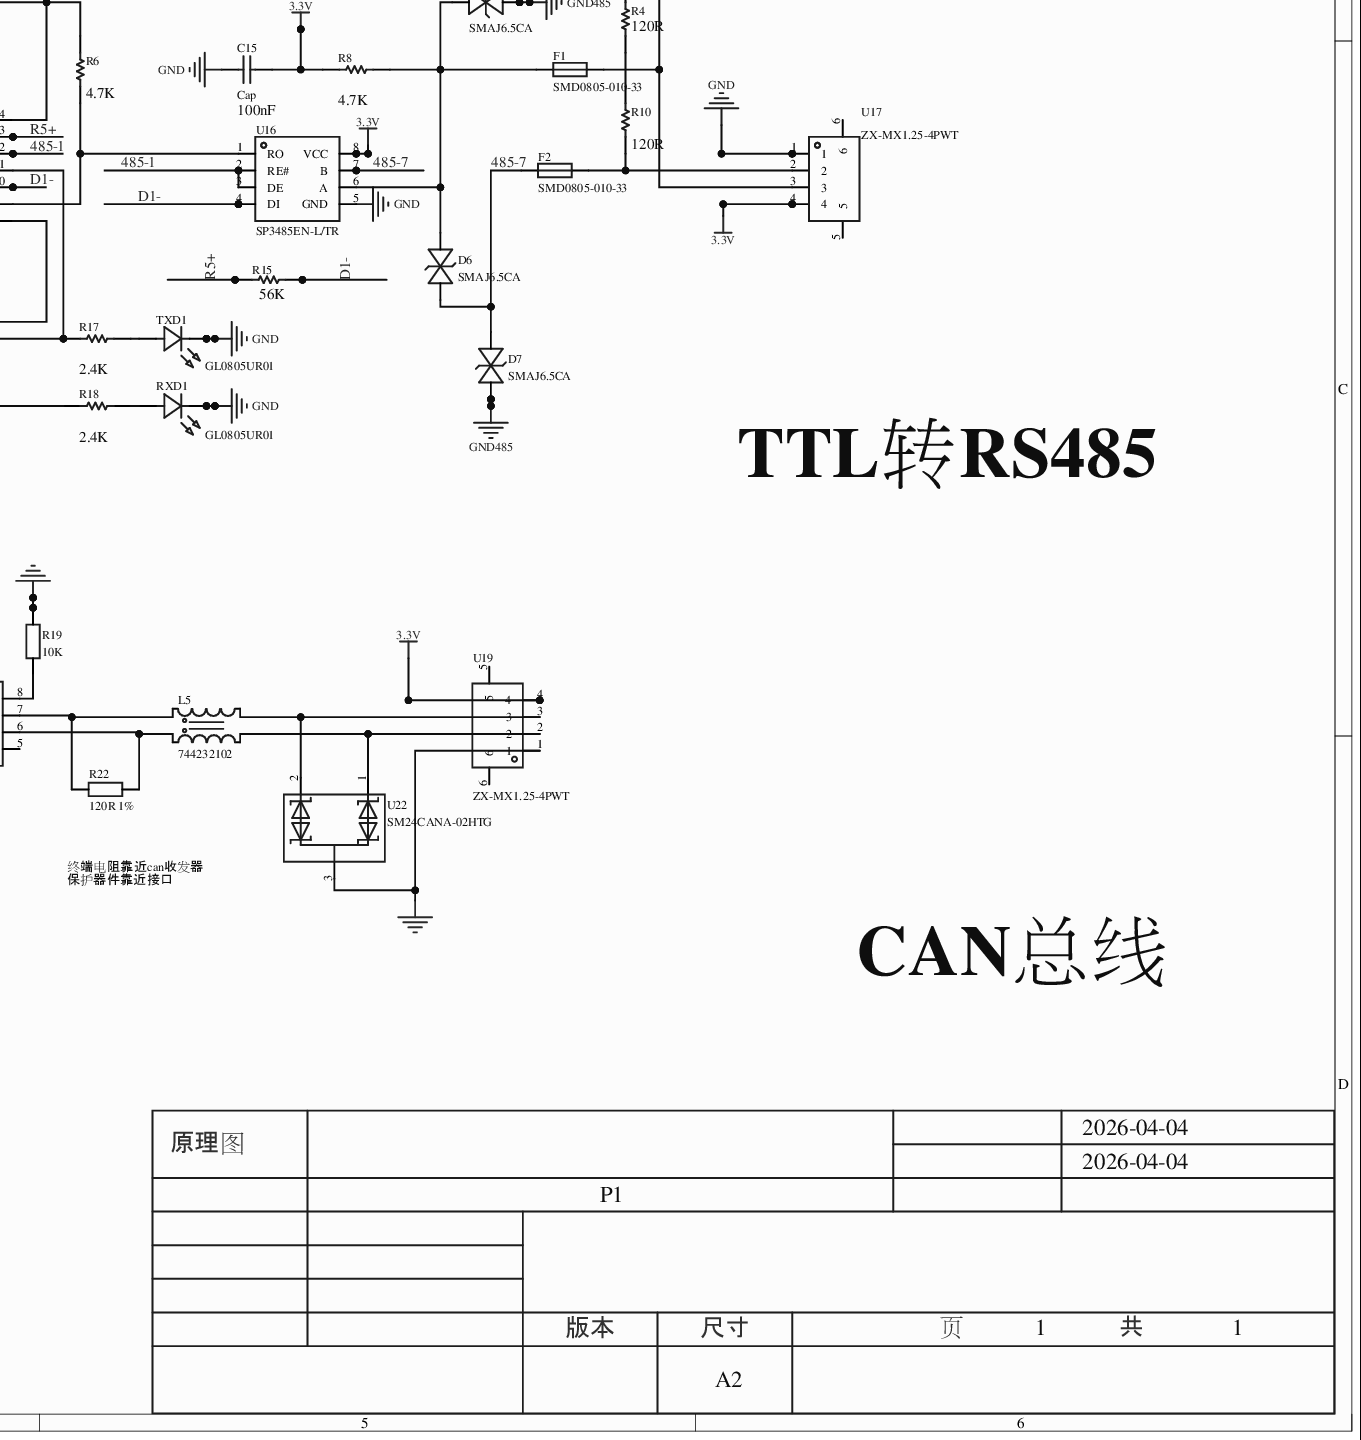
[diagram p0: MISC51972-3.schdoc, bottom right]
# Altium project MISC51972-2.PrjPcb (part 3 of 3)

## Sheet MISC51972-3.schdoc (continued)

### Library data of the parts
C1 C3 C4 C6-C8 = CAP_0402: SymbolName: CapAcitance; ConvertToPcb: yes; ModelId: 36a51122f27c49738f86b3bfa98863e0; ModelName: C0402_L1.0-W0.5-H0.5; ModelTransform: 39.37,19.685,0,0,0,0,0,0,0; Device: CAP_0402; FootprintName: C0402; AddInBom: yes; Supplier Footprint: 0402; Value: 100nF
C2 C5 C9-C14 C16-C20 C27 C28 C35 C36 = CAP_0603: SymbolName: CapAcitance; ConvertToPcb: yes; ModelId: ac125912035d415993ca9572d50418b1; ModelName: C0603_L1.6-W0.8-H0.8; ModelTransform: 62.992,31.496,0,0,0,0,0,0,0; Device: CAP_0603; FootprintName: C0402; AddInBom: yes; Supplier Footprint: 0603
  C2 C5 C11-C14 C16-C20: Value: 100nF
  C9 C10: Value: 12pF
  C27 C35: Value: 10uF
  C28 C36: Value: 22uF
C15 C21 = Cap: Capacitor; Origin Footprint: C0603; AddInBom: yes; ModelId: fca5be93b99f4b5a9a2fd372d58c31d9; ModelTransform: 0,0,0,0,0,0,0,0,0; Device: Cap; Symbol: Cap; Design Item ID: Cap; Library Name: Miscellaneous Devices; Published: 8-Jun-2000; LatestRevisionDate: 17-Jul-2002; LatestRevisionNote: Re-released for DXP Platform.; PackageReference: RAD-0.3; PackageDescription: Radial Cap, Thru-Hole; 2 Leads; 0.3 in Pin Spacing; FootprintName: C0402; ConvertToPcb: yes; ModelName: C0603; Publisher: Altium Limited
C22 C25 = CC0603KRX7R9BB104: 容值:100nF;精度:±10%;额定电压:50V;温度系数:X7R;; Manufacturer: YAGEO(国巨); AddInBom: yes; Tolerance: ±10%; Voltage Rating: 50V; Temperature Coefficient: X7R; ModelId: ac125912035d415993ca9572d50418b1; ModelName: C0603_L1.6-W0.8-H0.8; ModelTransform: 62.992,31.496,0,0,0,0,0,0,0; Device: CC0603KRX7R9BB104; Symbol: CC0603KRX7R9BB104; FootprintName: C0402; LCSC Part Name: 100nF ±10% 50V; SupplierPart: C14663; ManufacturerPart: CC0603KRX7R9BB104; Supplier Footprint: 0603; JLCPCB Part Class: 基础库; Datasheet: https://item.szlcsc.com/datasheet/CC0603KRX7R9BB104/15331.html; Supplier: LCSC; ConvertToPcb: yes; Value: 100nF
C23 C24 = CGA0603X5R226M100JT: 容值:22uF;精度:±20%;额定电压:10V;温度系数:X5R;; Manufacturer: HRE(芯声); AddInBom: yes; Tolerance: ±20%; Voltage Rating: 10V; Temperature Coefficient: X5R; ModelId: ac125912035d415993ca9572d50418b1; ModelName: C0603_L1.6-W0.8-H0.8; ModelTransform: 62.992,31.496,0,0,0,0,0,0,0; Device: CGA0603X5R226M100JT; Symbol: CGA0603X5R226M100JT; FootprintName: C0402; LCSC Part Name: 22uF ±20% 10V; SupplierPart: C6119863; ManufacturerPart: CGA0603X5R226M100JT; Supplier Footprint: 0603; JLCPCB Part Class: 扩展库; Datasheet: https://item.szlcsc.com/datasheet/CGA0603X5R226M100JT/7062569.html; Supplier: LCSC; ConvertToPcb: yes; Value: 22uF
C29 C34 = CL10B104KB8NNNC: 容值:100nF;精度:±10%;额定电压:50V;材质(温度系数):X7R;; Manufacturer: SAMSUNG(三星); AddInBom: yes; Tolerance: ±10%; Voltage Rated: 50V; Temperature Coefficient: X7R; ModelId: ac125912035d415993ca9572d50418b1; ModelName: C0603_L1.6-W0.8-H0.8; ModelTransform: 62.992,31.496,0,0,0,0,0,0,0; Device: CL10B104KB8NNNC; Symbol: CL10B104KB8NNNC; Supplier: LCSC; Manufacturer Part: CL10B104KB8NNNC; Value: 100nF; Supplier Part: C1591; JLCPCB Part Class: Extended Part; FootprintName: C0603; LCSC Part Name: 100nF ±10% 50V; Supplier Footprint: 0603; Datasheet: https://atta.szlcsc.com/upload/public/pdf/source/20160103/1457707680512.pdf; ConvertToPcb: yes
C30 = GRM31CR61E476ME44L: 容值:47uF;精度:±20%;额定电压:25V;材质(温度系数):X5R;; Manufacturer: muRata(村田); AddInBom: yes; Tolerance: ±20%; Voltage Rated: 25V; Temperature Coefficient: X5R; ModelId: e4be705b945545a48e666415e3682bd8; ModelName: C1206_L3.2-W1.6-H1.3; ModelTransform: 125.984,62.992,0,0,0,0,0,0,0; Device: GRM31CR61E476ME44L; Symbol: GRM31CR61E476ME44L; Supplier: LCSC; Supplier Part: C403725; Manufacturer Part: GRM31CR61E476ME44L; Value: 47uF; JLCPCB Part Class: Extended Part; FootprintName: C1206; LCSC Part Name: 47uF ±20% 25V; Supplier Footprint: 1206; Datasheet: https://atta.szlcsc.com/upload/public/pdf/source/20191025/C403725_B8A8CD2FFA1F57E6FDF268BD106459D5.pdf; ConvertToPcb: yes
C31 = M2221M025C090RT: 类型:聚合物;容值:220uF;精度:±20%;额定电压:25V;纹波电流:2.1A@100kHz;等效串联电阻:50mΩ@100kHz;; Manufacturer: 瑞隆; AddInBom: yes; Type: 聚合物; Tolerance: ±20%; Rated Voltage: 25V; Lifetime @ Temp: 2000hrs@105℃; ModelId: c6b4664e433d40ca9637ce321a5ed5ca; ModelTransform: 283.464,255.905,0,0,0,0,0,0,0; Device: M2221M025C090RT; Symbol: M2221M025C090RT; FootprintName: CAP-SMD_BD6.3-L6.5-W6.5-LS7.2-FD; LCSC Part Name: 220uF ±20% 25V; SupplierPart: C2898864; ManufacturerPart: M2221M025C090RT; Supplier Footprint: SMD,6.3x9mm; JLCPCB Part Class: Extended Part; Datasheet: https://atta.szlcsc.com/upload/public/pdf/source/20211011/C2898288_DE75CBD7B89218235B2C66F86F8FAB88.pdf; Supplier: LCSC; ConvertToPcb: yes; Value: 220uF; φD: -; L: -; Lead Spacing: -; Ripple Current: 2.1A@100kHz; Equivalent Series Resistance(ESR): 50mΩ@100kHz; Operating Temperature: -55℃~+105℃; ModelName: CAP-SMD_BD6.3-L6.5-W6.5-LS7.2-FD
C32 = SVZ1VM101E09E00RAXXX: 类型:聚合物;容值:100uF;精度:±20%;额定电压:35V;纹波电流:-;等效串联电阻:-;; Manufacturer: AISHI(艾华集团); AddInBom: yes; Type: 聚合物; Tolerance: ±20%; Rated Voltage: 35V; φD: 6.3mm; L: 9mm; ModelId: da0aaf7be69940018ee0d2811560c3a5; ModelTransform: 255.905,275.59,0,90,0,0,0,0,0; Device: SVZ1VM101E09E00RAXXX; Symbol: SVZ1VM101E09E00RAXXX; Supplier: LCSC; Supplier Part: C2939795; Manufacturer Part: SVZ1VM101E09E00RAXXX; Value: 100uF; JLCPCB Part Class: Extended Part; FootprintName: CAP-SMD_BD6.3-L6.5-W6.5-LS7.0-FD; LCSC Part Name: 100uF ±20% 35V; Supplier Footprint: SMD,6.3x9mm; Datasheet: https://atta.szlcsc.com/upload/public/pdf/source/20220111/A7F51B4B57636E51FA8F936B9D146736.pdf; ConvertToPcb: yes; Lead Spacing: -; Ripple Current: -; Equivalent Series Resistance(ESR): -; Lifetime @ Temp: -; Operating Temperature: -55℃~+105℃; ModelName: CAP-SMD_BD6.3-L6.5-W6.5-LS7.0-FD
C33 = CL31B475KBHNNNE: 容值:4.7uF;精度:±10%;额定电压:50V;材质(温度系数):X7R;; Manufacturer: SAMSUNG(三星); AddInBom: yes; Tolerance: ±10%; Voltage Rated: 50V; Temperature Coefficient: X7R; ModelId: e4be705b945545a48e666415e3682bd8; ModelName: C1206_L3.2-W1.6-H1.3; ModelTransform: 125.984,62.992,0,0,0,0,0,0,0; Device: CL31B475KBHNNNE; Symbol: CL31B475KBHNNNE; Supplier: LCSC; Manufacturer Part: CL31B475KBHNNNE; Value: 4.7uF; Supplier Part: C51205; JLCPCB Part Class: Extended Part; FootprintName: C0603; LCSC Part Name: 4.7uF ±10% 50V; Supplier Footprint: 1206; Datasheet: https://atta.szlcsc.com/upload/public/pdf/source/20160103/1457707732693.pdf; ConvertToPcb: yes
C37 = MT18B472K500CT: 容值:4.7nF;精度:±10%;额定电压:50V;材质(温度系数):X7R;; Manufacturer: Walsin(华新科); AddInBom: yes; Tolerance: ±10%; Voltage Rated: 50V; Temperature Coefficient: X7R; ModelId: ac125912035d415993ca9572d50418b1; ModelName: C0603_L1.6-W0.8-H0.8; ModelTransform: 62.992,31.496,0,0,0,0,0,0,0; Device: MT18B472K500CT; Symbol: MT18B472K500CT; Supplier: LCSC; Supplier Part: C366882; Manufacturer Part: MT18B472K500CT; Value: 4.7nF; JLCPCB Part Class: 扩展库; FootprintName: C0603; LCSC Part Name: 4.7nF ±10% 50V; Supplier Footprint: 0603; Datasheet: https://atta.szlcsc.com/upload/public/pdf/source/20190225/C366882_E806E7D8175088070BA62B5811C10C1A.pdf; ConvertToPcb: yes
D1-D4 = CD143A-SR05: 极性:单向;反向截止电压(Vrwm):5V;最大钳位电压:20V;峰值脉冲电流(Ipp):30A@8/20us;峰值脉冲功率(Ppp):500W;击穿电压:6V;; Manufacturer: BOURNS; AddInBom: yes; polarity: 单向; Reverse Stand-Off Voltage (Vrwm): 5V; Maximum Clamping Voltage: 20V; Peak Pulse Power Dissipation (Ppp): 500W; Breakdown Voltage: 6V; Type: TVS; ModelId: 2f65c54dcf124ea98761abb8aba517da; ModelTransform: 91.04793,118.11,0,270,0,0,0,0,0; Device: CD143A-SR05; Symbol: CD143A-SR05; FootprintName: SOT-143_L2.9-W1.3-P1.92-LS2.3-BL; LCSC Part Name: CD143A-SR05; SupplierPart: C840639; ManufacturerPart: CD143A-SR05; Supplier Footprint: SOT-143; JLCPCB Part Class: 扩展库; Datasheet: https://atta.szlcsc.com/upload/public/pdf/source/20240126/B7D1DDCC218735B2484CC455B566484D.pdf; Supplier: LCSC; ConvertToPcb: yes; Peak Pulse Current (Ipp): 30A@8/20us; ModelName: SOT-143_L2.9-W1.3-P1.92-LS2.3-BL
D5-D7 = SMAJ6.5CA_C19077527: 极性:双向;反向截止电压(Vrwm):6.5V;钳位电压:11.2V;峰值脉冲电流(Ipp):35.7A@10/1000us;峰值脉冲功率(Ppp):400W@10/1000us;击穿电压:7.98V;; Manufacturer: R+O(宏嘉诚); AddInBom: yes; Polarity: 双向; Reverse Stand-Off Voltage (Vrwm): 6.5V; Clamping Voltage: 11.2V; Voltage - Breakdown: 7.98V; Reverse Leakage Current (Ir): 500uA; Number of Channels: 单路; level of protection: IEC 61000-4-2; Type: TVS; ModelId: 158e58edd1c6495db0cdb6a8ba85866f; ModelTransform: 208.661,105.1179,0,0,0,0,0,0,0; Device: SMAJ6.5CA_C19077527; Symbol: SMAJ6.5CA_C19077527; FootprintName: SMA-L4.3-W2.6-LS5.3-BI; LCSC Part Name: 双向TVS 6.5V截止 峰值浪涌电流：35.7A@10/1000us; SupplierPart: C19077527; ManufacturerPart: SMAJ6.5CA; Supplier Footprint: DO-214AC(SMA); JLCPCB Part Class: 扩展库; Datasheet: https://item.szlcsc.com/datasheet/SMAJ6.5CA/20275612.html; Supplier: LCSC; ConvertToPcb: yes; Peak Pulse Current (Ipp): 35.7A@10/1000us; Peak Pulse Power Dissipation (Ppp): 400W@10/1000us; Operating Temperature: -55℃~+150℃; Junction Capacitance: -; ModelName: SMA-L4.3-W2.6-LS5.3-BI
D8 = LL4148_C435829: 二极管配置:-;正向压降(Vf):1V@10mA;直流反向耐压(Vr):75V;整流电流:200mA;反向恢复时间(Trr):4ns;; Manufacturer: MDD(辰达半导体); AddInBom: yes; Voltage - DC Reverse(Vr): 75V; Current - Rectified: 200mA; Pd - Power Dissipation: 500mW; Reverse Leakage Current (Ir): 5uA@75V; Reverse Recovery Time (trr): 4ns; Non-Repetitive Peak Forward Surge Current: 4A; ModelId: 4a6f2309ca4c4217857da1816cccdf69; ModelName: LL-34_L3.5-W1.5; ModelTransform: 133.93674,59.031,0,0,0,0,0,0,0; Device: LL4148_C435829; Symbol: LL4148_C435829; FootprintName: LL-34_L3.5-W1.5-RD; LCSC Part Name: 75V 200mA; SupplierPart: C435829; ManufacturerPart: LL4148; Supplier Footprint: LL-34; JLCPCB Part Class: 扩展库; Datasheet: https://item.szlcsc.com/datasheet/LL4148/433090.html; Supplier: LCSC; ConvertToPcb: yes; Diode Configuration: -; Voltage - Forward(Vf@If): 1V@10mA; Operating Junction Temperature Range: -
D9 D10 = SS54_C513478: 直流反向耐压(Vr):40V;平均整流电流(Io):5A;正向压降(Vf):550mV@5A;; Manufacturer: Slkor(萨科微); AddInBom: yes; Reverse Voltage (Vr): 40V; Average Rectified Current (Io): 5A; ModelId: 228de99b63224bd3982b21290755dd84; ModelTransform: 204.724,110.236,0,0,0,0,0,0,0; Device: SS54_C513478; Symbol: SS54_C513478; Supplier: LCSC; Supplier Part: C513478; Manufacturer Part: SS54; JLCPCB Part Class: Extended Part; FootprintName: SMA_L4.4-W2.8-LS5.4-R-RD; LCSC Part Name: 40V 5A 550mV@5A; Supplier Footprint: SMA; Datasheet: https://atta.szlcsc.com/upload/public/pdf/source/20200414/C513471_6461A1BCB05B602A4F47401B394AA5A8.pdf; ConvertToPcb: yes; Forward Voltage (Vf@If): 550mV@5A; ModelName: SMA_L4.4-W2.8-LS5.4-R-RD
DC1 = DC-005-A200: 连接器类型:DC电源插座;安装方式:弯插;触点内径:2mm;触点外径:6.4mm;额定电流:3A;额定电压:30V;工作温度:-20℃~+70℃;; Manufacturer: XUNPU(讯普); AddInBom: yes; Connector Type: DC电源插座; Inside Contact Diameter: 2mm; Outside Contact Diameter: 6.4mm; Current Rating: 3A; Voltage Rating (Max): 30V; ModelId: 1321cdbe1dc84555a9684967491c8670; ModelTransform: 553.149,368.14887,0,0,0,0,-137.795,85.63,-161.417; Device: DC-005-A200; Symbol: DC-005-A200; FootprintName: DC-IN-TH_DC-005-A200; LCSC Part Name: DC电源插座 内径:2mm 外径:6.4mm; SupplierPart: C720557; ManufacturerPart: DC-005-A200; Supplier Footprint: 插件; JLCPCB Part Class: 扩展库; Datasheet: https://item.szlcsc.com/datasheet/DC-005-A200/763564.html; Supplier: LCSC; ConvertToPcb: yes; Mounting Type: 弯插; Operating Temperature: -20℃~+70℃; ModelName: DC-IN-TH_DC-005-A200
F1 F2 = SMD0805-010-33: 耐压(Vmax):33V;最大电流(Imax):40A;保持电流(Ihold):100mA;跳闸电流(Itrip):300mA;; Manufacturer: R+O(宏嘉诚); AddInBom: yes; Voltage - Max: 33V; Current - Max: 40A; Hold Current: 100mA; Trip Current: 300mA; Power Dissipation: 500mW; Resistance - Initial (Ri) (Min): 750mΩ; Resistance - Post Trip (R1) (Max): 6Ω; Time to Trip(Max): 500ms; ModelId: 57e2aa106f9143e8b6ab832aebb31c78; ModelName: F0805_L2.1-W1.4-H0.8; ModelTransform: 82.677,55.118,0,0,0,0,0.0005,0,0; Device: SMD0805-010-33; Symbol: SMD0805-010-33; FootprintName: F0805; LCSC Part Name: SMD0805-010-33; SupplierPart: C46640975; ManufacturerPart: SMD0805-010-33; Supplier Footprint: 0805; JLCPCB Part Class: 扩展库; Datasheet: https://item.szlcsc.com/datasheet/SMD0805-010-33/48798681.html; Supplier: LCSC; ConvertToPcb: yes; Operating Temperature: -40℃~+85℃; Length: 2.2mm; Width: 1.5mm; Height: 0.9mm
H1 H2 = PZ254V-11-04P: 插针结构:1x4P;间距:2.54mm;行距:-;圆针/方针:方针;安装方式:直插;排数:单排;总PIN位数:4P;额定电流:3A;额定电压:250V;配合针长度:6mm;塑高:2.5mm;端接针长度:3mm;触头材质:-;工作温度:-40℃~+105℃;颜色:黑色;; Manufacturer: XFCN(兴飞); Symbol: PZ254V-11-04P_C2691448; AddInBom: yes; Pin Structure: 1x4P; Pitch: 2.54mm; Circluar Pins/Square Pins: 方针; Current Rating: 3A; Voltage Rating (Max): 250V; ModelId: 112f4d05e8d64e99ab9a333894bea4f9; ModelName: HDR-TH_4P-P2.54-M-LI-1X4P; ModelTransform: 399.999,104.7242,0,0,0,0,0,0,-118.11; Device: PZ254V-11-04P; FootprintName: HDR-TH_4P-P2.54-V-M; LCSC Part Name: 1x4P 间距:2.54mm 方针 直插; SupplierPart: C2691448; ManufacturerPart: PZ254V-11-04P; Supplier Footprint: 插件,P=2.54mm; JLCPCB Part Class: 扩展库; Datasheet: https://item.szlcsc.com/datasheet/PZ254V-11-04P/2801085.html; Supplier: LCSC; ConvertToPcb: yes; Row Spacing: -; Mounting Type: 直插; Number of Rows: 单排; Number of Pins: 4P; Length of Mating Pin: 6mm; Insulation Height: 2.5mm; Length of End Connection Pin: 3mm; Contact Material: -; Operating Temperature: -40℃~+105℃; Color: 黑色
L1-L4 = DLM11SN900HY2L: 通道数:2;阻抗@频率:90Ω@100MHz;直流电阻(DCR):1.38Ω;; Manufacturer: muRata(村田); AddInBom: yes; Number of Lines: 2; Voltage Withstand: 12.5V; Current Rating: 100mA; Voltage Rating - DC: 5V; DC Resistance(DCR): 1.38Ω; Insulation Resistance(IR): 100MΩ; ModelId: 1f3893ab612b4e86bdc6b0aad8b614a6; ModelName: SMD-4_L1.3-W1.0-H0.9-P0.55; ModelTransform: 50,39.37,0,0,0,0,0,0,0; Device: DLM11SN900HY2L; Symbol: DLM11SN900HY2L; FootprintName: FILTER-SMD_4P-L1.3-W1.0-TL_DLP11SN201HL2L; LCSC Part Name: 停产 两路 贴片共模滤波器 阻抗90Ω@100MHz Min，电源线滤波; SupplierPart: C161089; ManufacturerPart: DLM11SN900HY2L; Supplier Footprint: SMD-4P,1.2x1mm; JLCPCB Part Class: 扩展库; Datasheet: https://item.szlcsc.com/datasheet/DLM11SN900HY2L/172470.html; Supplier: LCSC; ConvertToPcb: yes; Impedance @ Frequency: 90Ω@100MHz; Operating Temperature: -40℃~+85℃
L5 = 744232102: 通道数:2;电感@频率:1.263uH;阻抗@频率:1kΩ@100MHz;直流电阻(DCR):1Ω;; Manufacturer: Wurth(伍尔特); AddInBom: yes; Number of Lines: 2; Current Rating: 230mA; Voltage Rating - DC: 50V; Voltage Withstand: 125V; DC Resistance(DCR): 1Ω; ModelId: e90643789ecb4eb1904e019ee2202aaa; ModelName: IND-SMD_4P-L3.2-W1.6-H1.9; ModelTransform: 125.984,62.992,0,0,0,0,0,0,0; Device: 744232102; Symbol: 744232102; FootprintName: IND-SMD_4P-L3.2-W1.6; LCSC Part Name: 1 kΩ @ 100MHz 230mA; SupplierPart: C2662336; ManufacturerPart: 744232102; Supplier Footprint: SMD-4P,3.2x1.6mm; JLCPCB Part Class: 扩展库; Datasheet: https://www.we-online.com/components/products/datasheet/744232102.pdf; Supplier: LCSC; ConvertToPcb: yes; Inductance @ Frequency: 1.263uH; Impedance @ Frequency: 1kΩ@100MHz; Operating Temperature: -40℃~+125℃
L6 = FXL0630-3R3-M: 电感值:3.3uH;精度:±20%;额定电流:8.5A;饱和电流(Isat):9.5A;类型:一体成型电感;; Manufacturer: cjiang(长江微电); AddInBom: yes; Tolerance: ±20%; Rated Current: 8.5A; Saturation Current (Isat): 9.5A; DC Resistance (DCR): 22mΩ; Type: 一体成型电感; ModelId: 6860c29aec394a38a0f014af7f722a42; ModelName: IND-SMD_L7.0-W6.6-H3.0; ModelTransform: 275.59,259.88137,0,0,0,0,0,0,0; Device: FXL0630-3R3-M; Symbol: FXL0630-3R3-M; FootprintName: IND-SMD_L7.0-W6.6; LCSC Part Name: 3.3uH ±20% 9.5A; SupplierPart: C167219; ManufacturerPart: FXL0630-3R3-M; Supplier Footprint: SMD,6.6x7mm; JLCPCB Part Class: 扩展库; Datasheet: https://atta.szlcsc.com/upload/public/pdf/source/20240426/3189EA8206330E2108542F9E34E540E7.pdf; Supplier: LCSC; ConvertToPcb: yes; Value: 3.3uH
L7 = MWSA0624S-4R7MT: 类型:-;电感值:4.7uH;精度:±20%;额定电流:5A;饱和电流(Isat):6.5A;; Manufacturer: Sunlord(顺络); AddInBom: yes; Tolerance: ±20%; Saturation Current (Isat): 6.5A; DC Resistance (DCR): 50mΩ; ModelId: 6860c29aec394a38a0f014af7f722a42; ModelName: IND-SMD_L7.0-W6.6-H3.0; ModelTransform: 275.59,259.88137,0,0,0,0,0,0,0; Device: MWSA0624S-4R7MT; Symbol: MWSA0624S-4R7MT; FootprintName: IND-SMD_L7.0-W6.6; LCSC Part Name: 4.7uH ±20% 6.5A; SupplierPart: C408433; ManufacturerPart: MWSA0624S-4R7MT; Supplier Footprint: SMD; JLCPCB Part Class: 扩展库; Datasheet: https://atta.szlcsc.com/upload/public/pdf/source/20190729/C408433_59F7EFF54638F38A6E803A8FCE4E2CFD.pdf; Supplier: LCSC; ConvertToPcb: yes; Type: -; Value: 4.7uH; Ratings: -
LED1 = 15-21VGC/TR8: 照明颜色:普绿/黄绿;色温 - CCT（K）:-;主波长/色坐标:571nm;; Manufacturer: EVERLIGHT(亿光); AddInBom: yes; Illumination Color: 普绿/黄绿; Luminous Intensity (IF=20mA): 13mcd; Dominant Wavelength / Coordinate rank: 571nm; ModelId: 9925348f94944448bd3e9ceb708e7ae9; ModelName: LED1206_Inf; ModelTransform: 118.11,59.055,0,180,0,0,0,0,0; Device: 15-21VGC/TR8; Symbol: 15-21VGC/TR8; FootprintName: LED0603_GREEN; LCSC Part Name: 发光二极管1206普绿/黄绿; SupplierPart: C131289; ManufacturerPart: 15-21VGC/TR8; Supplier Footprint: 1206; JLCPCB Part Class: Extended Part; Datasheet: https://atta.szlcsc.com/upload/public/pdf/source/20170918/C131289_1505726897595976297.pdf; Supplier: LCSC; ConvertToPcb: yes; Mounting Type: 表面贴装; Correlated Color Temperature - CCT(K): -; Luminous Flux/Radiant Flux: -
R1-R3 R7 R9 R11-R14 R19 R22 = Res_0603: SymbolName: 电阻; ConvertToPcb: yes; ModelId: fc143cca1e79419f9cd78b61e9279f08; ModelName: R0603; ModelTransform: 31.8897,63.7794,0,90,0,0,0,0,0; Device: Res_0603; FootprintName: R0402; AddInBom: yes; Supplier Footprint: 0603
  R1 R2: Value: 0R
  R3: Value: 9.53K
  R7: Value: 90.9K
  R9 R19: Value: 10K
  R11-R14: Value: 4.7K
  R22: Value: 120R 1%
R4-R6 R8 R10 R15-R18 = Res1: Resistor; Origin Footprint: R0603; AddInBom: yes; ModelId: fc143cca1e79419f9cd78b61e9279f08; ModelTransform: 31.8897,63.7794,0,90,0,0,0,0,0; Device: Res1; Symbol: Res1; Design Item ID: Res1; Library Name: Miscellaneous Devices; Published: 8-Jun-2000; LatestRevisionDate: 17-Jul-2002; LatestRevisionNote: Re-released for DXP Platform.; PackageReference: AXIAL-0.3; PackageDescription: Axial Device, Thru-Hole; 2 Leads; 0.3 in Pin Spacing; FootprintName: R0402; ConvertToPcb: yes; ModelName: R0603; Publisher: Altium Limited
R20 R23 = 0603WAF1002T5E: 电阻类型:厚膜电阻;阻值:10kΩ;精度:±1%;功率:100mW;工作电压:75V;温度系数:±100ppm/℃;; Manufacturer: UNI-ROYAL(厚声); AddInBom: yes; Tolerance: ±1%; Power(Watts): 100mW; Voltage-Supply(Max): 75V; ModelId: fc143cca1e79419f9cd78b61e9279f08; ModelName: R0603; ModelTransform: 31.8897,63.7794,0,90,0,0,0,0,0; Device: 0603WAF1002T5E; Symbol: 0603WAF1002T5E; FootprintName: R0402; LCSC Part Name: 厚膜电阻 10kΩ ±1% 100mW; SupplierPart: C25804; ManufacturerPart: 0603WAF1002T5E; Supplier Footprint: 0603; JLCPCB Part Class: 基础库; Datasheet: https://item.szlcsc.com/datasheet/0603WAF1002T5E/26547.html; Supplier: LCSC; ConvertToPcb: yes; Type: 厚膜电阻; Value: 10kΩ; Temperature Coefficient: ±100ppm/℃; Operating Temperature: -55℃~+155℃
R21 = 0603WAF4301T5E: 电阻类型:厚膜电阻;阻值:4.3kΩ;精度:±1%;功率:100mW;工作电压:75V;温度系数:±100ppm/℃;; Manufacturer: UNI-ROYAL(厚声); AddInBom: yes; Tolerance: ±1%; Power(Watts): 100mW; Voltage-Supply(Max): 75V; ModelId: fc143cca1e79419f9cd78b61e9279f08; ModelName: R0603; ModelTransform: 31.8897,63.7794,0,90,0,0,0,0,0; Device: 0603WAF4301T5E; Symbol: 0603WAF4301T5E; FootprintName: R0402; LCSC Part Name: 4.3kΩ ±1% 100mW 厚膜电阻; SupplierPart: C23159; ManufacturerPart: 0603WAF4301T5E; Supplier Footprint: 0603; JLCPCB Part Class: 扩展库; Datasheet: https://item.szlcsc.com/datasheet/0603WAF4301T5E/23886.html; Supplier: LCSC; ConvertToPcb: yes; Type: 厚膜电阻; Value: 4.3kΩ; Temperature Coefficient: ±100ppm/℃; Operating Temperature: -55℃~+155℃
R24-R29 = RC0603FR-074K7L: 阻值:4.7kΩ;精度:±1%;功率:100mW;温度系数:±100ppm/℃;最大工作电压:75V;工作温度范围:-55℃~+155℃;; Manufacturer: YAGEO(国巨); AddInBom: yes; Tolerance: ±1%; Power(Watts): 100mW; Overload Voltage (Max): 75V; ModelId: 6bd5cd867e9542ebae21caaf5d2d4c4d; ModelName: R0603; ModelTransform: 31.8897,63.7794,0,90,0,0,0,0,0; Device: RC0603FR-074K7L; Symbol: RC0603FR-074K7L; FootprintName: R0402; LCSC Part Name: 4.7kΩ ±1% 100mW; ManufacturerPart: RC0603FR-074K7L; Supplier Footprint: 0603; JLCPCB Part Class: Extended Part; Datasheet: https://atta.szlcsc.com/upload/public/pdf/source/20171030/C99782_15093665213961068236.pdf; Supplier: LCSC; ConvertToPcb: yes; Temperature Coefficient: ±100ppm/℃; Operating Temperature Range: -55℃~+155℃
  R24: Value: 51kΩ
  R25: Value: 4.7kΩ
  R26: Value: 1.5kΩ
  R27: Value: 200kΩ
  R28: Value: 10kΩ
  R29: Value: 20kΩ
RXD1 TXD1 = GL0805UR01: 发光颜色:红色;正向压降(Vf):2.1V;正向电流:10mA;波长:618nm~624nm;二极管配置:独立二极管;透镜颜色:无色透明透镜;发光强度:100mcd;发光角度:120°;载带方式:正贴;工作温度:-40℃~+85℃;; Manufacturer: Guiguang light(桂光光电); AddInBom: yes; Illumination Color: 红色; Voltage - Forward(Vf): 2.1V; Forward Current: 10mA; Diode Configuration: 独立二极管; Lens Color: 无色透明透镜; Luminous Intensity: 100mcd; Viewing Angle: 120°; ModelId: f010e90d36544999ab4e363fdba5b490; ModelTransform: 78.74,49.21644,0,0,0,0,0,0,0; Device: GL0805UR01; Symbol: GL0805UR01; FootprintName: LED0805-R-RD_RED; LCSC Part Name: 0805 红灯 高亮; SupplierPart: C51933307; ManufacturerPart: GL0805UR01; Supplier Footprint: 0805; JLCPCB Part Class: 扩展库; Datasheet: https://item.szlcsc.com/datasheet/GL0805UR01/54646003.html; Supplier: LCSC; ConvertToPcb: yes; Wavelength - Dominant: 618nm~624nm; Mounting Style: 正贴; Operating Temperature: -40℃~+85℃; ModelName: LED0805-R-RD_RED
U1 U7 = TXS0102DCUT: 数据速率:24Mbps;工作电压(VCCA):1.65V~3.6V;工作电压(VCCB):2.3V~5.5V;通道数:1;每个电路通道数:2;; Manufacturer: TI(德州仪器); AddInBom: yes; Channel Type: 双向; Data Rate: 24Mbps; Number of Circuits: 2; Output Type: 开漏；推挽式; ModelId: c85411b4a3544d83a02d075c4dadd21f; ModelName: VSSOP-8_L2.3-W2.0-P0.50-LS3.1-BL; ModelTransform: 78.74,122.047,0,90,0,0,0,0,0; Device: TXS0102DCUT; Symbol: TXS0102DCUT; FootprintName: VSSOP-8_L2.3-W2.0-P0.50-LS3.1-BR; LCSC Part Name: 24Mbps 2位双向电平转换器; SupplierPart: C2655478; ManufacturerPart: TXS0102DCUT; Supplier Footprint: VSSOP-8-0.5mm; JLCPCB Part Class: 扩展库; Datasheet: https://www.ti.com/cn/lit/gpn/txs0102; Supplier: LCSC; ConvertToPcb: yes; Input Signal: -; Output Signal: -; Voltage - Supply(VCCA): 1.65V~3.6V; Voltage - Supply(VCCB): 2.3V~5.5V; Operating Temperature: -40℃~+85℃; Features: 自动方向检测
U2 U8 = TPS2060CDGNR: 通道数:2;输出电流:1.5A;输入电压:4.5V~5.5V;导通电阻:70mΩ;; Manufacturer: TI(德州仪器); AddInBom: yes; Number of Outputs: 2; Output Current: 1.5A; Resistor On-State: 70mΩ; ModelId: 5bbd78b5ce6a42cb9dc58d1e47c0e385; ModelTransform: 118.11,192.913,0,0,0,0,0,0,0; Device: TPS2060CDGNR; Symbol: TPS2060CDGNR; FootprintName: HVSSOP-8_L3.0-W3.0-P0.65-LS4.9-BL-EP-1; LCSC Part Name: TPS2060CDGNR; SupplierPart: C2149825; ManufacturerPart: TPS2060CDGNR; Supplier Footprint: MSOP-8; JLCPCB Part Class: 扩展库; Datasheet: https://www.ti.com/cn/lit/gpn/tps2066c; Supplier: LCSC; ConvertToPcb: yes; Input Voltage: 4.5V~5.5V; Operating Temperature	-: -40℃~+125℃; ModelName: HVSSOP-8_L3.0-W3.0-P0.65-LS4.9-BL-EP-1
U3 U5 U9 U11 = PCMF2USB3S: AddInBom: yes; Device: PCMF2USB3S; SymbolName: PCMF2USB3S; FootprintName: PCMF2USB3S; ConvertToPcb: yes
U4 U6 U10 U12 = tp点: AddInBom: yes; Device: tp点; SymbolName: tp点; FootprintName: tp点; ConvertToPcb: yes
U13 = HC-USB3.0-L168-WP: 连接器类型:Type-A;协议标准:USB 3.0;公母:母;安装方式:弯插;触点数量:9P;端口数量:1;额定电流 - 电源:1.5A;工作温度:-25℃~+70℃;; Manufacturer: HC(虹成电子); AddInBom: yes; Connector Type: Type-A; Protocol Standard: USB 3.0; Gender: 母; Number of Contacts: 9P; Number of Ports: 1; Current Rating-Power: 1.5A; Voltage Rating: 30V; Connect-Disconnect Life: 1.5千次; Detection color: 蓝色; ModelId: a6994728bee34198bb5c5e1920a86239; ModelTransform: 614.14546,661.41998,0,0,0,0,-0.001,-204.724,-137.795; Device: HC-USB3.0-L168-WP; Symbol: HC-USB3.0-L168-WP; FootprintName: USB-TH_USB3.0-A; LCSC Part Name: Type-A 母 弯插 USB3.0 A母90度 弯脚蓝色平口 吸塑盒; SupplierPart: C7501850; ManufacturerPart: HC-USB3.0-L168-WP; Supplier Footprint: 弯插; JLCPCB Part Class: 扩展库; Datasheet: https://item.szlcsc.com/datasheet/HC-USB3.0-L168-WP/8585391.html; Supplier: LCSC; ConvertToPcb: yes; Mounting Type: 弯插; Supplementary Features: -; Center Height: -; Length: 16.8mm; Operating Temperature: -25℃~+70℃; ModelName: USB-TH_USB3.0-A
U14 = TUSB8041IRGCR: TUSB8041 TUSB8041 四端口 USB 3.0 集线器; Manufacturer: TI(德州仪器); AddInBom: yes; USB Protocol: USB 3.0；USB 2.0; Voltage - Supply: 0.99V~1.26V；3V~3.6V; Memory Interface: I2C；SMBus; Current - Supply: 778mA; Supply Current (Iq): 33mA; Number of Channels: 4; ModelId: bd201a332e104d48be6c84c32c9d6f8d; ModelName: QFN-64_L9.0-W9.0-H1.0-P0.50; ModelTransform: 354.331,354.332,0,90,0,0,0,0,0; Device: TUSB8041IRGCR; Symbol: TUSB8041IRGCR; FootprintName: QFN-64_L9.0-W9.0-P0.50-BL-EP7.2; LCSC Part Name: TUSB8041IRGCR; SupplierPart: C544686; ManufacturerPart: TUSB8041IRGCR; Supplier Footprint: QFN-64-EP(9x9); JLCPCB Part Class: 扩展库; Datasheet: https://www.ti.com/cn/lit/gpn/tusb8041; Supplier: LCSC; ConvertToPcb: yes; type: 集线器; Operating Temperature: -40℃~+85℃
U15 = 74HC04D,653: 输入类型:-;工作电压:2V~6V;静态电流(Iq):2uA;通道数:6;传播延迟(tpd):14ns@6V,50pF;; Manufacturer: Nexperia(安世); AddInBom: yes; Voltage - Supply: 2V~6V; Quiescent Current(Iq): 2uA; Number of Circuits: 6; Number of Inputs: 1; Current - Output Low(IOL): 5.2mA; Input Logic Level - High: 1.5V~4.2V; Input Logic Level -Low: 500mV~1.8V; Output Logic Level - High: 3.7V；5.2V；1.9V; Output Logic Level - Low: 400mV；400mV；100mV; ModelId: 8dbf5b715d42428c85558507ae5a252b; ModelName: SOIC-14_L8.6-W3.9-H1.8-LS6.0-P1.27; ModelTransform: 338.583,236.22,0,0,0,0,0,0.001,0; Device: 74HC04D,653; Symbol: 74HC04D,653; FootprintName: SOIC-14_L8.7-W3.9-P1.27-LS6.0-BL; LCSC Part Name: 六路反相器; SupplierPart: C5590; ManufacturerPart: 74HC04D,653; Supplier Footprint: SOIC-14; JLCPCB Part Class: 扩展库; Datasheet: https://item.szlcsc.com/datasheet/74HC04D%252C653/6041.html; Supplier: LCSC; ConvertToPcb: yes; Input Type: -; Current - Output High(IOH): 5.2mA; Propagation Delay: 14ns@6V,50pF; Series: 74HC系列; Operating Temperature: -40℃~+125℃
U16 = SP3485EN-L/TR: 类型:收发器;数据速率:10Mbps;; Manufacturer: MaxLinear(迈凌); AddInBom: yes; Number of Drivers: 1; Voltage - Supply: 3.3V; Data Rate: 10Mbps; Number of Nodes: 32; Supply Current (Iq): 2mA; Communication Mode: 半双工; ModelId: 7abc64c95a1a4a04a4ef38f9097c870b; ModelTransform: 192.913,236.22,0,0,0,0,0,0,0; Device: SP3485EN-L/TR; Symbol: SP3485EN-L/TR; FootprintName: SOIC-8_L5.0-W4.0-P1.27-LS6.0-BL; LCSC Part Name: SP3485 +3.3V低功耗半双工RS-485收发器，数据速率10Mbps; SupplierPart: C8963; ManufacturerPart: SP3485EN-L/TR; Supplier Footprint: SOIC-8; JLCPCB Part Class: 基础库; Datasheet: https://item.szlcsc.com/datasheet/SP3485EN-L%252FTR/9482.html; Supplier: LCSC; ConvertToPcb: yes; Type: 收发器; Number of Receivers: 1; Operating Temperature: -40℃~+85℃; ModelName: SOIC-8_L5.0-W4.0-P1.27-LS6.0-BL
U17 U19 = ZX-MX1.25-4PWT: 插针结构:1x4P;间距:1.25mm;安装方式:卧贴;参考系列:PicoBlade(MX 1.25);总PIN数:4P;排数:1;每排PIN数:4;行距:-;额定电流:1A;触头材质:黄铜;触头镀层:锡;工作温度:-25℃~+85℃;; Manufacturer: Megastar(兆星); AddInBom: yes; Pins Structure: 1x4P; Pitch: 1.25mm; Number of PINs Per Row: 4; Current Rating: 1A; Voltage Rating: 125V; Plastic Material: LCP; Supplementary Features: 辅助焊脚; Z-Height of the Board: 3.6mm; X-Length of Bottom Edge on Board (Spacing Line): 10mm; Y-Width of Bottom Edge on Board: 5.25mm; ModelId: 71b205b306fe40bda91ecc831d13606d; ModelTransform: 395.6685,208.661,0,0,0,0,0,-32.951,0; Device: ZX-MX1.25-4PWT; Symbol: ZX-MX1.25-4PWT; FootprintName: CONN-SMD_4P-P1.25-MX1.25-4P-WT; LCSC Part Name: 1x4P 间距:1.25mm 卧贴 系列:PicoBlade(MX 1.25); SupplierPart: C7430470; ManufacturerPart: ZX-MX1.25-4PWT; Supplier Footprint: SMD,P=1.25mm,卧贴; JLCPCB Part Class: 扩展库; Datasheet: https://item.szlcsc.com/datasheet/ZX-MX1.25-4PWT/8430339.html; Supplier: LCSC; ConvertToPcb: yes; Mounting Type: 卧贴; Reference Series: PicoBlade(MX 1.25); Number of Pins: 4P; Number of Rows: 1; Row Spacing: -; Contact Material: 黄铜; Contact Plating: 锡; Operating Temperature: -25℃~+85℃; Flame Retardant Rating: -; Color: 米色; ModelName: CONN-SMD_4P-P1.25-MX1.25-4P-WT
U18 = SN65HVD230DR: 类型:CAN收发器;数据速率:1Mbps;; Manufacturer: TI(德州仪器); AddInBom: yes; Data Rate: 1Mbps; ModelId: e81d2f7d937b4a6ab1dca543ff5d56a4; ModelName: SOIC-8_L4.9-W3.9-H1.7-LS6.0-P1.27; ModelTransform: 192.913,236.22,0,0,0,0,0,0,0; Device: SN65HVD230DR; Symbol: SN65HVD230DR; FootprintName: SOIC-8_L4.9-W3.9-P1.27-LS6.0-BL; LCSC Part Name: 3.3-V CAN 收发器; SupplierPart: C12084; ManufacturerPart: SN65HVD230DR; Supplier Footprint: SOIC-8; JLCPCB Part Class: 扩展库; Datasheet: https://www.ti.com/cn/lit/gpn/sn65hvd230; Supplier: LCSC; ConvertToPcb: yes; Type: CAN收发器; Voltage - Supply: -; Current - Supply: -; Operating Temperature: -40℃~+85℃
U20 = AMS1117-1.8_C6185: 输出类型:固定;工作电压:15V;输出电压:1.8V;输出电流:1A;电源纹波抑制比(PSRR):72dB@(120Hz);输出极性:正极;; Manufacturer: AMS; AddInBom: yes; Output Type: 固定; Voltage - Supply: 15V; Output Voltage: 1.8V; Output Current: 1A; Voltage Dropout: 1.3V@(1A); Noise: 0.003%Vout; Output Configuration: 正极; Number of Outputs: 1; ModelId: 925194bf9823436183a3e0b978a8d076; ModelName: SOT-223-4P_L6.5-W3.5-H1.6-LS7.0-P2.30; ModelTransform: 279.89794,255.905,0,180,0,0,-0.0005,-0.0005,0; Device: AMS1117-1.8_C6185; Symbol: AMS1117-1.8; FootprintName: SOT-223-4_L6.5-W3.5-P2.30-LS7.0-BR; LCSC Part Name: 输入15V 输出1.8V 1A; SupplierPart: C6185; ManufacturerPart: AMS1117-1.8; Supplier Footprint: SOT-223; JLCPCB Part Class: 扩展库; Datasheet: https://item.szlcsc.com/datasheet/AMS1117-1.8/6651.html; Supplier: LCSC; ConvertToPcb: yes; Power Supply Rejection Ratio (PSRR): 72dB@(120Hz); Features: 短路保护；过热保护; Operating Temperature: -40℃~+125℃@(Tj)
U21 = TPS563201DDCR: 功能类型:降压型;输出类型:可调;工作电压:4.5V~17V;输出电压:768mV~7V;输出电流:3A;; Manufacturer: TI(德州仪器); AddInBom: yes; Function: 降压型; Output Type: 可调; Output Current: 3A; Frequency - Switching: 580kHz; Synchronous Rectifier: 是; Number of Outputs: 1; Topology: 降压式; Switch tube (built-in/external): 内置; ModelId: 18da8f6c14a34920b3e136b5c401a119; ModelName: SOT-23-6_L2.9-W1.6-H1.5-LS2.8-P0.95; ModelTransform: 110.73671,114.173,0,180,0,0,0.001,-0.003,0; Device: TPS563201DDCR; Symbol: TPS563201DDCR; FootprintName: SOT-23-6_L2.9-W1.6-P0.95-LS2.8-BR; LCSC Part Name: 4.5V至17V输入，3A同步降压电压调节器; SupplierPart: C116592; ManufacturerPart: TPS563201DDCR; Supplier Footprint: SOT-23-THIN-6; JLCPCB Part Class: 扩展库; Datasheet: https://item.szlcsc.com/datasheet/TPS563201DDCR/117846.html; Supplier: LCSC; ConvertToPcb: yes; Voltage - Supply: 4.5V~17V; Output Voltage: 768mV~7V; Operating Temperature: -40℃~+125℃@(TJ); Quiescent Current: -
U22 = SM24CANA-02HTG_C2936979: 极性:双向;反向截止电压(Vrwm):24V;钳位电压:40V;峰值脉冲电流(Ipp):4A;峰值脉冲功率(Ppp):140W;击穿电压:26.7V;; Manufacturer: TECH PUBLIC(台舟); AddInBom: yes; Polarity: 双向; Reverse Stand-Off Voltage (Vrwm): 24V; Clamping Voltage: 40V; Peak Pulse Current (Ipp): 4A; Peak Pulse Power Dissipation (Ppp): 140W; Voltage - Breakdown: 26.7V; Reverse Leakage Current (Ir): 80nA; Number of Channels: 双路; level of protection: IEC 61000-4-4；IEC 61000-4-5；IEC 61000-4-2; Junction Capacitance: 10pF；7pF; ModelId: c62791f0466c4ae2a892c056b845b0ca; ModelName: SOT-23-3P_L2.9-W1.3-H1.0-LS2.4-P0.95; ModelTransform: 98.425,114.173,0,180,0,0,0.0005,-0.0005,0; Device: SM24CANA-02HTG_C2936979; Symbol: SM24CANA-02HTG_C2936979; FootprintName: SOT-23-3_L2.9-W1.3-P1.90-LS2.4-BR; LCSC Part Name: 双向 24V截止 峰值浪涌电流：4A; SupplierPart: C2936979; ManufacturerPart: SM24CANA-02HTG; Supplier Footprint: SOT-23; JLCPCB Part Class: 扩展库; Datasheet: https://item.szlcsc.com/datasheet/SM24CANA-02HTG/3290326.html; Supplier: LCSC; ConvertToPcb: yes; Operating Temperature: -55℃~+125℃
U23 = SCT2450STER: Manufacturer: SCT(芯洲科技); AddInBom: yes; ModelId: d3e00daa36c445139c055a3b9efb85d2; ModelName: ESOP-8_L4.9-W3.9-H1.6-LS6.0-P1.27; ModelTransform: 240.157,192.913,0,90,0,0,0,0,0; Device: SCT2450STER; Symbol: SCT2450STER; FootprintName: ESOP-8_L4.9-W3.9-P1.27-LS6.0-BL-EP; LCSC Part Name: 电源IC; SupplierPart: C509400; ManufacturerPart: SCT2450STER; Supplier Footprint: ESOP-8; JLCPCB Part Class: 扩展库; Datasheet: https://atta.szlcsc.com/upload/public/pdf/source/20200407/C509400_EDF779A672A59398CFBA9E95FA584FEC.pdf; Supplier: LCSC; ConvertToPcb: yes
U24 = AMS1117-3.3_C347222: 输出类型:固定;工作电压:12V;输出电压:3.3V;输出电流:1A;电源纹波抑制比(PSRR):60dB@(120Hz);输出极性:正极;; Manufacturer: UMW(友台半导体); AddInBom: yes; Output Type: 固定; Voltage - Supply: 12V; Output Voltage: 3.3V; Output Current: 1A; Voltage Dropout: 1.3V@(1A); standby current: 5mA; Noise: 0.003%Vout; Output Configuration: 正极; Number of Outputs: 1; ModelId: 925194bf9823436183a3e0b978a8d076; ModelName: SOT-223-4P_L6.5-W3.5-H1.6-LS7.0-P2.30; ModelTransform: 279.89794,255.905,0,180,0,0,-0.0005,-0.0005,0; Device: AMS1117-3.3_C347222; Symbol: AMS1117-3.3_C347222; FootprintName: SOT-223-4_L6.5-W3.5-P2.30-LS7.0-BR; LCSC Part Name: 3.3V 1A 12V; SupplierPart: C347222; ManufacturerPart: AMS1117-3.3; Supplier Footprint: SOT-223; JLCPCB Part Class: 扩展库; Datasheet: https://item.szlcsc.com/datasheet/AMS1117-3.3/323882.html; Supplier: LCSC; ConvertToPcb: yes; Power Supply Rejection Ratio (PSRR): 60dB@(120Hz); Features: 过流保护; Operating Temperature: -40℃~+125℃
USB1 USB2 = HC-USB3.0-L175-2X1-P: 连接器类型:Type-A;协议标准:USB 3.0;公母:母;安装方式:弯插;触点数量:9Px2;端口数量:2;额定电流 - 电源:1.5A;工作温度:-;; Manufacturer: HC(虹成电子); AddInBom: yes; Connector Type: Type-A; Protocol Standard: USB 3.0; Gender: 母; Number of Contacts: 9Px2; Number of Ports: 2; Current Rating-Power: 1.5A; Voltage Rating: 30V; Detection color: 蓝色; ModelId: 4c0a715a39bf464c8af9d479827ed79e; ModelTransform: 616.91944,678.811,0,0,0,0,0,-163.386,-137.795; Device: HC-USB3.0-L175-2X1-P; Symbol: HC-USB3.0-L175-2X1-P; FootprintName: USB-A-TH_H181-AF2R06-12ALCR; LCSC Part Name: Type-A 母 弯插 USB3.0 AF90度 双层短体17.5mm 弯脚平口蓝色; SupplierPart: C7501881; ManufacturerPart: HC-USB3.0-L175-2X1-P; Supplier Footprint: 弯插; JLCPCB Part Class: 扩展库; Datasheet: https://item.szlcsc.com/datasheet/HC-USB3.0-L175-2X1-P/8585422.html; Supplier: LCSC; ConvertToPcb: yes; Mounting Type: 弯插; Connect-Disconnect Life: -; Supplementary Features: -; Center Height: -; Length: 17.5mm; Operating Temperature: -; ModelName: USB-A-TH_H181-AF2R06-12ALCR
X1 = X322524MOB4SI: 晶振类型:贴片晶振;频率:24MHz;常温频差:±10ppm;负载电容:12pF;频率稳定度:±20ppm;; Manufacturer: YXC(扬兴晶振); AddInBom: yes; Normal temperature Frequency Tolerance: ±10ppm; Load Capacitance: 12pF; Frequency Stability: ±20ppm; ModelId: ff2dfd5650294453a14147960efe1838; ModelTransform: 125.984,98.425,0,0,0,0,0,0,0; Device: X322524MOB4SI; Symbol: X322524MOB4SI; FootprintName: CRYSTAL-SMD_4P-L3.2-W2.5-BL; LCSC Part Name: YSX321SL 24MHZ 4P 3225 12PF ±10PPM -40~85℃ (±20PPM); SupplierPart: C70590; ManufacturerPart: X322524MOB4SI; Supplier Footprint: SMD3225-4P; JLCPCB Part Class: 扩展库; Datasheet: https://item.szlcsc.com/datasheet/X322524MOB4SI/71688.html; Supplier: LCSC; ConvertToPcb: yes; Type: 贴片晶振; Value: 24MHz; Operating Temperature: -40℃~+85℃; ModelName: CRYSTAL-SMD_4P-L3.2-W2.5-BL